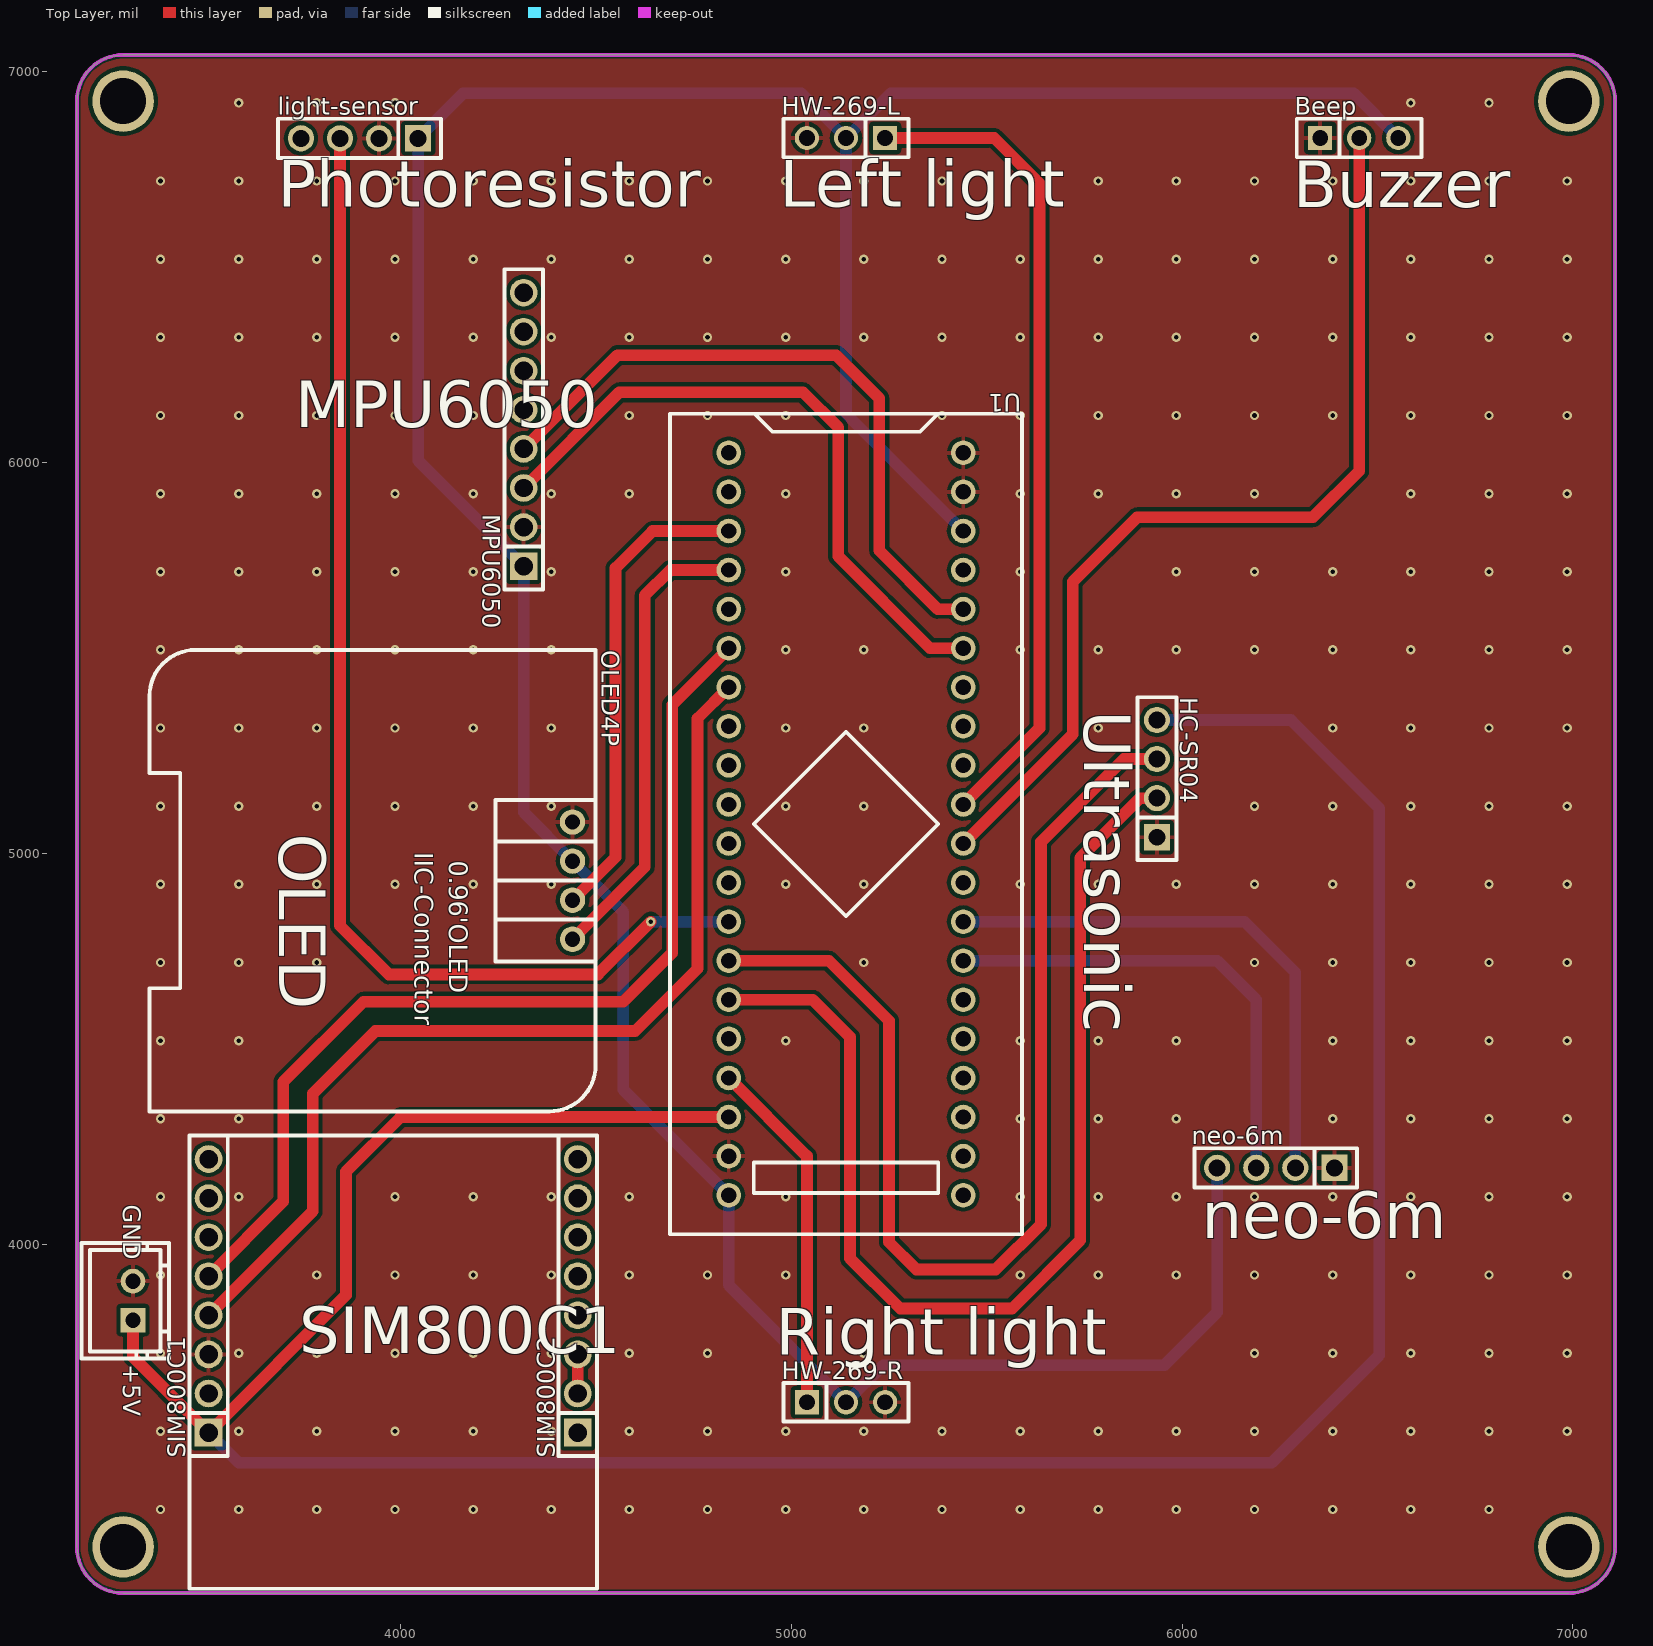
[diagram p0: Top Layer view]
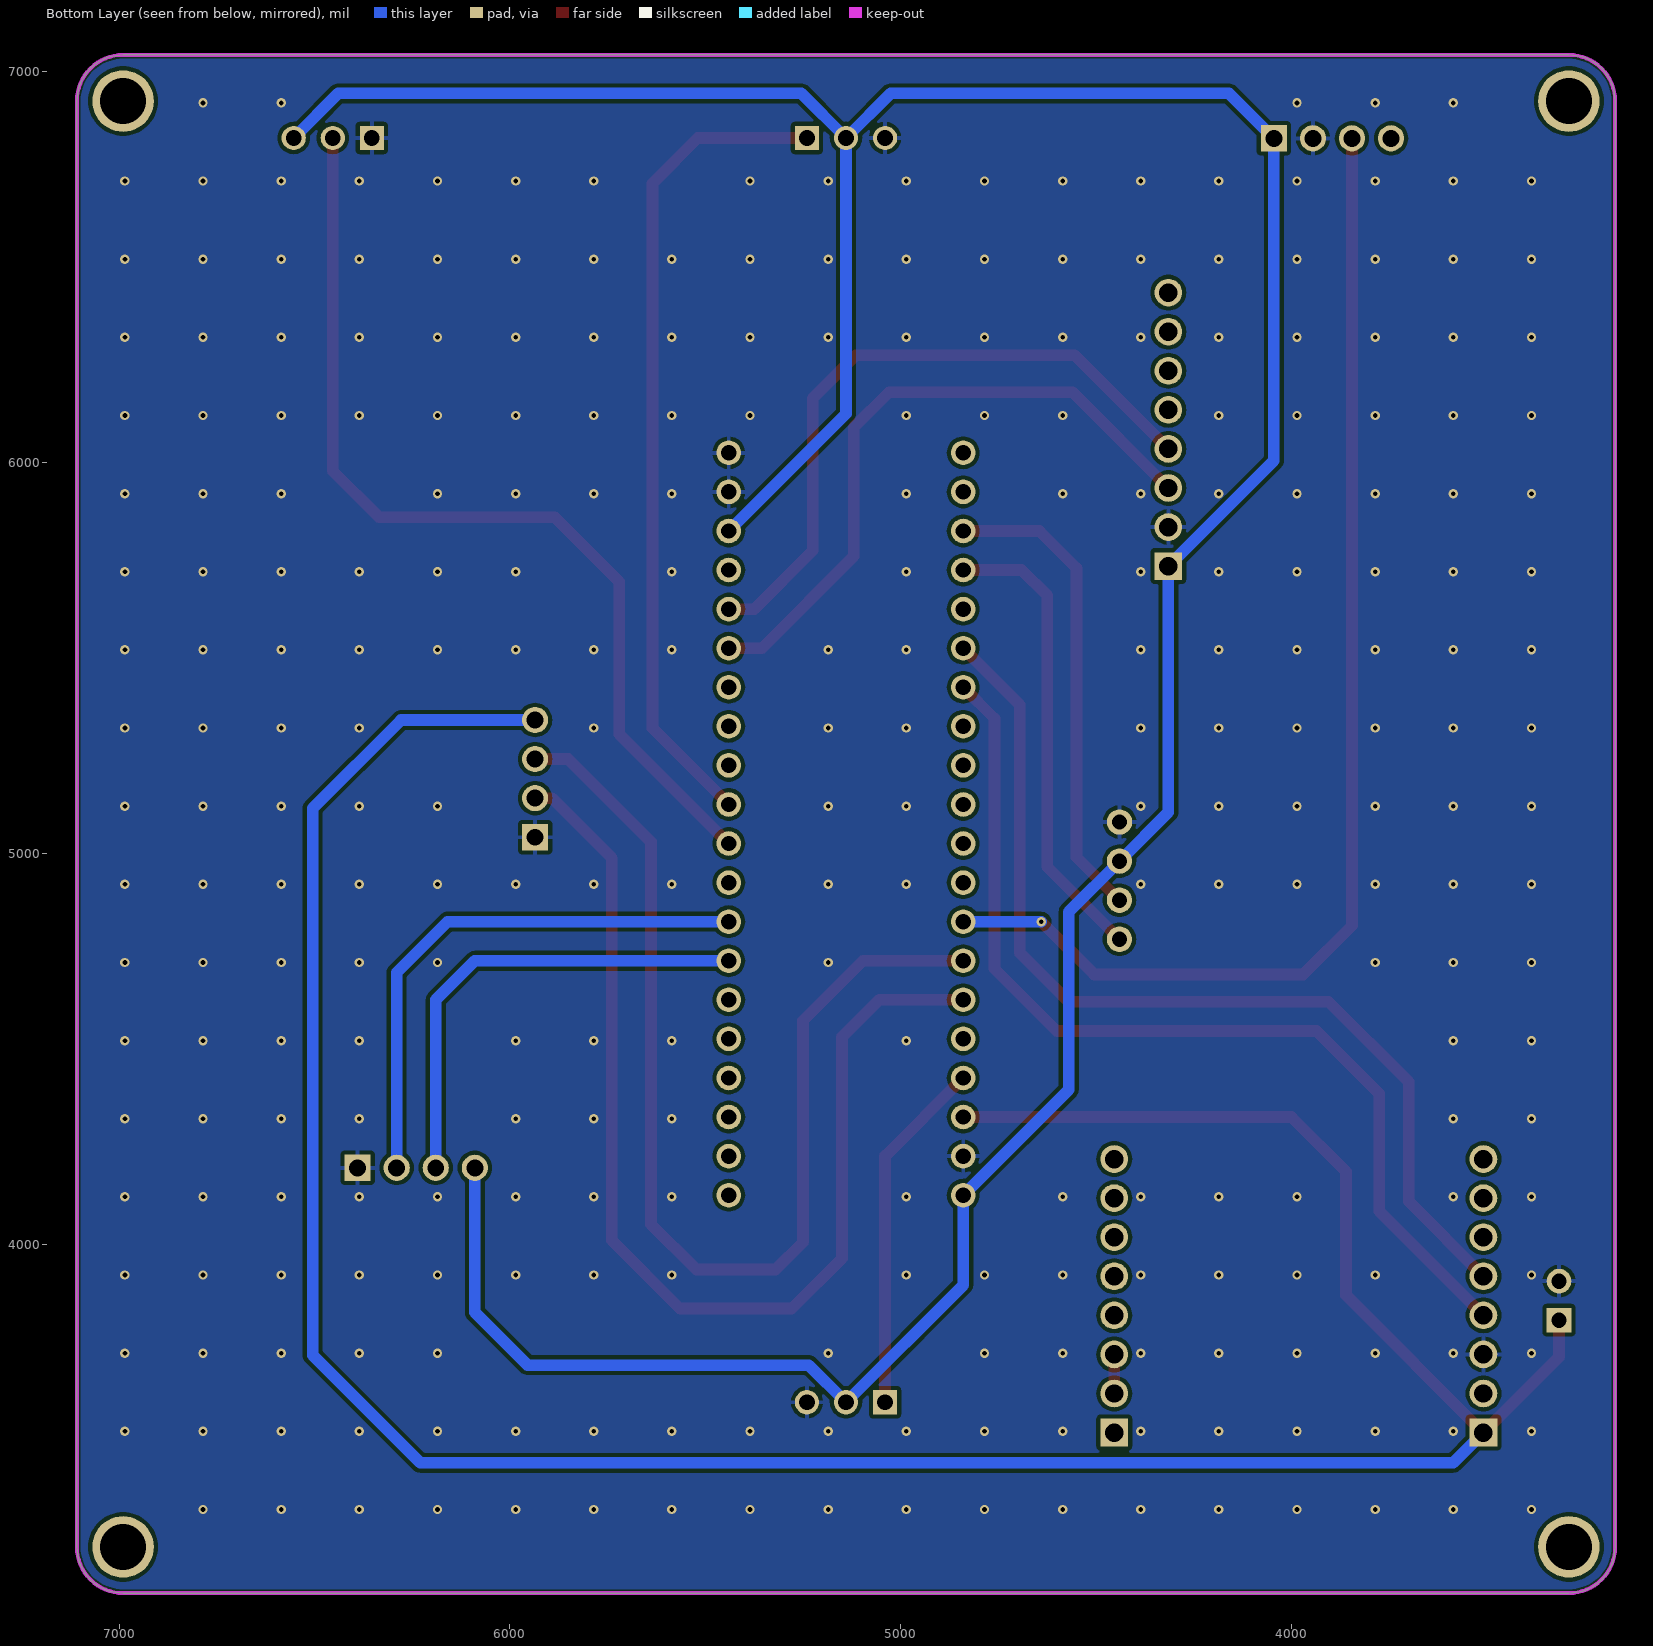
[diagram p1: Bottom Layer view, seen from below]
# Altium PCB MISC51587.pcbdoc
Units mil, origin at the board's own origin, x right, y up, seen from the top; angles counter-clockwise.
Board outline 3937.01 x 3937.01 mil, 2 copper layers (Top Layer, Bottom Layer), stack 62.206 mil thick; 12 components, 38 nets, 95 pads, 276 vias.

## Layer stack, top to bottom
Top Solder Mask Layer: solder mask 0.394, Dk 3.3
Top Layer: signal copper 1.379
Dielectric1: surface 59.449, FR4, Dk 4.5
Bottom Layer: signal copper 1.378
Bottom Solder Mask Layer: solder mask 0.394, Dk 3.3

## Board outline
6990.39,3106.5 ccw(c6990.39,3224.61) 7108.5,3224.61 7108.5,6925.39 ccw(c6990.39,6925.39) 6990.39,7043.5 3289.61,7043.5 ccw(c3289.61,6925.39) 3171.5,6925.39 3171.5,3224.61 ccw(c3289.61,3224.61) 3289.61,3106.5

## Design rules (kind name [scope] priority, off if disabled: settings)
BoardOutlineClearance copperThickness2oz_1 [All] p2 off: genericclearance=7.99 ignorepadtopadclearanceinfootprint=FALSE except(0: Arc-SplitContinuation Track-SplitContinuation SMDPad-SplitContinuation THPad-SplitContinuation Via-SplitContinuation Fill-SplitContinuation Region-SplitContinuation Poly-SplitContinuation Text-SplitContinuation Hole-SplitContinuation; 5.98: Arc-CutoutEdge Track-CutoutEdge SMDPad-CutoutEdge THPad-CutoutEdge Via-CutoutEdge Text-CutoutEdge; 6.89: Hole-OutlineEdge Hole-CutoutEdge; 10: Poly-OutlineEdge Poly-CutoutEdge; 11.81: Arc-OutlineEdge Track-OutlineEdge SMDPad-OutlineEdge THPad-OutlineEdge Via-OutlineEdge Fill-OutlineEdge Region-OutlineEdge Text-OutlineEdge Fill-CutoutEdge Region-CutoutEdge)
BoardOutlineClearance Plane_innerPlane_1 [All] p4 off: genericclearance=4.02 ignorepadtopadclearanceinfootprint=FALSE except(0: Arc-SplitContinuation Track-SplitContinuation SMDPad-SplitContinuation THPad-SplitContinuation Via-SplitContinuation Fill-SplitContinuation Region-SplitContinuation Poly-SplitContinuation Text-SplitContinuation Hole-SplitContinuation; 5.98: Arc-CutoutEdge Track-CutoutEdge SMDPad-CutoutEdge THPad-CutoutEdge Via-CutoutEdge Text-CutoutEdge; 6.89: Hole-OutlineEdge Hole-CutoutEdge; 10: Poly-OutlineEdge Poly-CutoutEdge; 11.81: Arc-OutlineEdge Track-OutlineEdge SMDPad-OutlineEdge THPad-OutlineEdge Via-OutlineEdge Fill-OutlineEdge Region-OutlineEdge Text-OutlineEdge Fill-CutoutEdge Region-CutoutEdge)
BoardOutlineClearance Copper_copperRegion_1 [All] p6 off: genericclearance=4.02 ignorepadtopadclearanceinfootprint=FALSE except(0: Arc-SplitContinuation Track-SplitContinuation SMDPad-SplitContinuation THPad-SplitContinuation Via-SplitContinuation Fill-SplitContinuation Region-SplitContinuation Poly-SplitContinuation Text-SplitContinuation Hole-SplitContinuation; 5.98: Arc-CutoutEdge Track-CutoutEdge SMDPad-CutoutEdge THPad-CutoutEdge Via-CutoutEdge Text-CutoutEdge; 6.89: Hole-OutlineEdge Hole-CutoutEdge; 10: Poly-OutlineEdge Poly-CutoutEdge; 11.81: Arc-OutlineEdge Track-OutlineEdge SMDPad-OutlineEdge THPad-OutlineEdge Via-OutlineEdge Fill-OutlineEdge Region-OutlineEdge Text-OutlineEdge Fill-CutoutEdge Region-CutoutEdge)
BoardOutlineClearance copperThickness1oz_1 [All] p8: genericclearance=4.02 ignorepadtopadclearanceinfootprint=FALSE except(0: Arc-SplitContinuation Track-SplitContinuation SMDPad-SplitContinuation THPad-SplitContinuation Via-SplitContinuation Fill-SplitContinuation Region-SplitContinuation Poly-SplitContinuation Text-SplitContinuation Hole-SplitContinuation; 5.98: Arc-CutoutEdge Track-CutoutEdge SMDPad-CutoutEdge THPad-CutoutEdge Via-CutoutEdge Text-CutoutEdge; 6.89: Hole-OutlineEdge Hole-CutoutEdge; 10: Poly-OutlineEdge Poly-CutoutEdge; 11.81: Arc-OutlineEdge Track-OutlineEdge SMDPad-OutlineEdge THPad-OutlineEdge Via-OutlineEdge Fill-OutlineEdge Region-OutlineEdge Text-OutlineEdge Fill-CutoutEdge Region-CutoutEdge)
Clearance copperThickness2oz [All] p1 off: gap=7.99 ignorepadtopadclearanceinfootprint=FALSE except(5.98: SMDPad-Track SMDPad-SMDPad THPad-Track SMDPad-THPad THPad-THPad Track-Via SMDPad-Via THPad-Via Via-Via Fill-SMDPad Region-SMDPad Fill-THPad Region-THPad Fill-Via Region-Via Fill-Fill Fill-Region Region-Region Arc-Track Arc-SMDPad Arc-THPad Arc-Via Fill-Arc Region-Arc Arc-Arc Text-Track SMDPad-Text Text-THPad Text-Via Fill-Text Region-Text Arc-Text Text-Text; 6.89: Hole-Track Hole-SMDPad Hole-THPad Hole-Via Fill-Hole Region-Hole Hole-Arc Hole-Text; 10: Poly-Track Poly-SMDPad Poly-THPad Poly-Via Poly-Fill Poly-Region Poly-Poly Poly-Arc Poly-Text Poly-Hole; 11.81: Fill-Track Region-Track)
Clearance Plane_innerPlane [All] p3 off: gap=4.02 ignorepadtopadclearanceinfootprint=FALSE except(5.98: SMDPad-Track SMDPad-SMDPad THPad-Track SMDPad-THPad THPad-THPad Track-Via SMDPad-Via THPad-Via Via-Via Fill-SMDPad Region-SMDPad Fill-THPad Region-THPad Fill-Via Region-Via Fill-Fill Fill-Region Region-Region Arc-Track Arc-SMDPad Arc-THPad Arc-Via Fill-Arc Region-Arc Arc-Arc Text-Track SMDPad-Text Text-THPad Text-Via Fill-Text Region-Text Arc-Text Text-Text; 6.89: Hole-Track Hole-SMDPad Hole-THPad Hole-Via Fill-Hole Region-Hole Hole-Arc Hole-Text; 10: Poly-Track Poly-SMDPad Poly-THPad Poly-Via Poly-Fill Poly-Region Poly-Poly Poly-Arc Poly-Text Poly-Hole; 11.81: Fill-Track Region-Track)
Clearance Copper_copperRegion [All] p5 off: gap=4.02 ignorepadtopadclearanceinfootprint=FALSE except(5.98: SMDPad-Track SMDPad-SMDPad THPad-Track SMDPad-THPad THPad-THPad Track-Via SMDPad-Via THPad-Via Via-Via Fill-SMDPad Region-SMDPad Fill-THPad Region-THPad Fill-Via Region-Via Fill-Fill Fill-Region Region-Region Arc-Track Arc-SMDPad Arc-THPad Arc-Via Fill-Arc Region-Arc Arc-Arc Text-Track SMDPad-Text Text-THPad Text-Via Fill-Text Region-Text Arc-Text Text-Text; 6.89: Hole-Track Hole-SMDPad Hole-THPad Hole-Via Fill-Hole Region-Hole Hole-Arc Hole-Text; 10: Poly-Track Poly-SMDPad Poly-THPad Poly-Via Poly-Fill Poly-Region Poly-Poly Poly-Arc Poly-Text Poly-Hole; 11.81: Fill-Track Region-Track)
Clearance copperThickness1oz [All] p7: gap=4.02 ignorepadtopadclearanceinfootprint=FALSE except(5.98: SMDPad-Track SMDPad-SMDPad THPad-Track SMDPad-THPad THPad-THPad Track-Via SMDPad-Via THPad-Via Via-Via Fill-SMDPad Region-SMDPad Fill-THPad Region-THPad Fill-Via Region-Via Fill-Fill Fill-Region Region-Region Arc-Track Arc-SMDPad Arc-THPad Arc-Via Fill-Arc Region-Arc Arc-Arc Text-Track SMDPad-Text Text-THPad Text-Via Fill-Text Region-Text Arc-Text Text-Text; 6.89: Hole-Track Hole-SMDPad Hole-THPad Hole-Via Fill-Hole Region-Hole Hole-Arc Hole-Text; 10: Poly-Track Poly-SMDPad Poly-THPad Poly-Via Poly-Fill Poly-Region Poly-Poly Poly-Arc Poly-Text Poly-Hole; 11.81: Fill-Track Region-Track)
DiffPairsRouting differentialPair [All] p1: maxlimit=6 minlimit=6 mostfreqgap=6 toplayer_minwidth=5 toplayer_prefwidth=10 toplayer_maxwidth=100 toplayer_mingap=6 toplayer_prefgap=6 toplayer_maxgap=6 bottomlayer_minwidth=5 bottomlayer_prefwidth=10 bottomlayer_maxwidth=100 bottomlayer_mingap=6 bottomlayer_prefgap=6 bottomlayer_maxgap=6 maxuncoupledlength=10
HoleToHoleClearance otherClearance [All] p1: gap=11.81 allowstackedmicrovias=TRUE
Length netLength [All] p1: minlimit=0 maxlimit=0
PasteMaskExpansion pasteMaskExpansion [All] p1: expansion=0
PlaneConnect innerPlane [All] p1: planeconnectstyle=Relief reliefexpansion=20 reliefentries=4 reliefconductorwidth=10 reliefairgap=10
PolygonConnect copperRegion [All] p1: connectstyle=Relief reliefconductorwidth=10 reliefentries=4 polygonreliefangle="90 Angle" airgapwidth=10 via.connectstyle=Relief via.reliefconductorwidth=10 via.reliefentries=4 via.polygonreliefangle="90 Angle" via.airgapwidth=10
RoutingVias viaSize [All] p1: holewidth=12.01 width=24.02 viastyle="Through Hole" minholewidth=11.81 minwidth=19.68 maxholewidth=248.03 maxwidth=393.7
SolderMaskExpansion solderMaskExpansion [IsVia] p1: expansion=-1000 istentingtop=TRUE
SolderMaskExpansion solderMaskExpansion [All] p2: expansion=2.01 istentingtop=FALSE
Width copperThickness2oz_2 [All] p1 off: maxlimit=100 minlimit=8 preferedwidth=10
Width copperThickness1oz_2 [All] p2: maxlimit=100 minlimit=5 preferedwidth=30

## Components (designator, comment, footprint, x,y, rotation, side; value= is the part's Value field where it differs from the comment)
+5V "_x001F_XH2.54-2P" CONN-TH_2P-P2.54-V 3315,3855 r90 top
Beep "" HDR-TH_3P-P2.54-V-F 6453.49,6830.79 r0 top
HC-SR04 "" HDR-TH_4P-P2.54-V-F 5935.69,5191.14 r90 top
HW-269-L "" HDR-TH_3P-P2.54-V-F 5140,6830.79 r180 top
HW-269-R "" HDR-TH_3P-P2.54-V-F 5140,3595 r0 top
light-sensor "" HDR-TH_4P-P2.54-V-F 3895,6830 r180 top
MPU6050 "" HDR-TH_8P-P2.54-V-F-1 4315,6085 r90 top
neo-6m "" HDR-TH_4P-P2.54-V-F 6240,4195 r180 top
OLED4P "" 0.96OLED_4P 4440,4930 r270 top
SIM800C1 "" HDR-TH_8P-P2.54-V-F-1 3508.5,3867.44 r90 top
SIM800C2 "" HDR-TH_8P-P2.54-V-F-1 4453.38,3867.44 r90 top
U1 "STM32F103C8T6-Card" CONN-TH_L53.3-W22.9_STM32F103C8T6-CARD 5140,5075 r270 top

## Footprints (in the part's own frame and the unit in brackets; to place one, negate y for a bottom-side part, rotate by r counter-clockwise, add the part's x,y. Pads: shape width x height; smd on the part's side, far side on the other; paste and mask are expansions set on the pad)
0.96OLED_4P [mm]
  round 1.65 hole 1 copper offset 0,0: 1(-3.81,-0.001) 2(-1.27,0.002) 3(1.27,0.002) 4(3.81,0.002)
  silkscreen extent -15,-27.5 15,1.5
CONN-TH_2P-P2.54-V [mm]
  rect 1.6x1.6 hole 1: 1(-1.27,0)
  round 1.6 hole 1: 2(1.27,0)
  silkscreen extent -3.75,-2.34 3.75,3.36
CONN-TH_L53.3-W22.9_STM32F103C8T6-CARD [mm]
  round 1.6 hole 1: 1(-24.13,-7.62) 2(-21.59,-7.62) 3(-19.05,-7.62) 4(-16.51,-7.62) 5(-13.97,-7.62) 6(-11.43,-7.62) 7(-8.89,-7.62) 8(-6.35,-7.62) 9(-3.81,-7.62) 10(-1.27,-7.62) 11(1.27,-7.62) 12(3.81,-7.62) 13(6.35,-7.62) 14(8.89,-7.62) 15(11.43,-7.62) 16(13.97,-7.62) 17(16.51,-7.62) 18(19.05,-7.62) 19(21.59,-7.62) 20(24.13,-7.62) 21(24.13,7.62) 22(21.59,7.62) 23(19.05,7.62) 24(16.51,7.62) 25(13.97,7.62) 26(11.43,7.62) 27(8.89,7.62) 28(6.35,7.62) 29(3.81,7.62) 30(1.27,7.62) 31(-1.27,7.62) 32(-3.81,7.62) 33(-6.35,7.62) 34(-8.89,7.62) 35(-11.43,7.62) 36(-13.97,7.62) 37(-16.51,7.62) 38(-19.05,7.62) 39(-21.59,7.62) 40(-24.13,7.62)
  silkscreen extent -26.67,-11.43 26.67,11.43
HDR-TH_3P-P2.54-V-F [mil]
  rect 62x62 hole 40.16: 1(-100,0)
  round 62 hole 40.16: 2(0,0) 3(100,0)
  silkscreen extent -160,-49 160,49
HDR-TH_4P-P2.54-V-F [mm]
  rect 1.7x1.7 hole 1.1: 1(-3.81,0)
  round 1.7 hole 1.1: 2(-1.27,0) 3(1.27,0) 4(3.81,0)
  silkscreen extent -5.29,-1.27 5.29,1.27
HDR-TH_8P-P2.54-V-F-1 [mm]
  rect 1.8x1.8 hole 1.2: 1(-8.89,0)
  round 1.8 hole 1.2: 2(-6.35,0) 3(-3.81,0) 4(-1.27,0) 5(1.27,0) 6(3.81,0) 7(6.35,0) 8(8.89,0)
  silkscreen extent -10.41,-1.25 10.41,1.25

## Free pads (board coordinates)
  round 157.48 hole 118.11: 1(3289.61,6925.39) 1(3289.61,3224.61) 1(6990.39,6925.39) 1(6990.39,3224.61)

## Via types
v1: diameter 24.02, hole 12, Top Layer to Bottom Layer, 276 vias

## Nets (pads, with @x,y where several pads share a name; then routed paths per layer and width w, separated by ;. In a path a pad name is that pad's centre, name@x,y a point inside that pad or via, vN(x,y) a via of type N, cw(c..) or ccw(c..) an arc to the next point about the centre after c; other vN are vias at no path point)
$1N18029: SIM800C2.2 SIM800C2.3 | length 100
  Top Layer w30: SIM800C2.2 SIM800C2.3
+5V: +5V.1 HC-SR04.4 SIM800C1.1 U1.18 | length 7424.3
  Top Layer w30: +5V.1 3315,3710.94 SIM800C1.1 3860,3868.94 3860,4185 4000,4325 U1.18
  Bottom Layer w30: SIM800C1.1 3585.94,3440 6230,3440 6505,3715 6505,5115 6278.86,5341.14 HC-SR04.4
GND: +5V.2 Beep.1 HC-SR04.1 HW-269-L.3 HW-269-R.3 light-sensor.2 MPU6050.2 neo-6m.1 OLED4P.1 SIM800C1.3 U1.19 U1.39 U1.40
  other v1: 3385.6,3320.6 3585.6,3320.6 3785.6,3320.6 3985.6,3320.6 4185.6,3320.6 4385.6,3320.6 4585.6,3320.6 4785.6,3320.6 4985.6,3320.6 5185.6,3320.6 5385.6,3320.6 5585.6,3320.6 5785.6,3320.6 5985.6,3320.6 6185.6,3320.6 6385.6,3320.6 6585.6,3320.6 6785.6,3320.6 3385.6,3520.6 3585.6,3520.6 3785.6,3520.6 3985.6,3520.6 4185.6,3520.6 4385.6,3520.6 4585.6,3520.6 4785.6,3520.6 4985.6,3520.6 5185.6,3520.6 5385.6,3520.6 5585.6,3520.6 5785.6,3520.6 5985.6,3520.6 6185.6,3520.6 6385.6,3520.6 6585.6,3520.6 6785.6,3520.6 6985.6,3520.6 3385.6,3720.6 3585.6,3720.6 3785.6,3720.6 3985.6,3720.6 4185.6,3720.6 4385.6,3720.6 4585.6,3720.6 4785.6,3720.6 5185.6,3720.6 6185.6,3720.6 6385.6,3720.6 6585.6,3720.6 6785.6,3720.6 6985.6,3720.6 3385.6,3920.6 3785.6,3920.6 3985.6,3920.6 4185.6,3920.6 4385.6,3920.6 4585.6,3920.6 4785.6,3920.6 4985.6,3920.6 5585.6,3920.6 5785.6,3920.6 5985.6,3920.6 6185.6,3920.6 6385.6,3920.6 6585.6,3920.6 6785.6,3920.6 6985.6,3920.6 3385.6,4120.6 3585.6,4120.6 3985.6,4120.6 4185.6,4120.6 4385.6,4120.6 4585.6,4120.6 4985.6,4120.6 5585.6,4120.6 5785.6,4120.6 5985.6,4120.6 6185.6,4120.6 6385.6,4120.6 6585.6,4120.6 6785.6,4120.6 6985.6,4120.6 3385.6,4320.6 3585.6,4320.6 5585.6,4320.6 5785.6,4320.6 5985.6,4320.6 6385.6,4320.6 6585.6,4320.6 6785.6,4320.6 6985.6,4320.6 3385.6,4520.6 3585.6,4520.6 4985.6,4520.6 5585.6,4520.6 5785.6,4520.6 5985.6,4520.6 6385.6,4520.6 6585.6,4520.6 6785.6,4520.6 6985.6,4520.6 3385.6,4720.6 3585.6,4720.6 3785.6,4720.6 5185.6,4720.6 6185.6,4720.6 6385.6,4720.6 6585.6,4720.6 6785.6,4720.6 6985.6,4720.6 3385.6,4920.6 3585.6,4920.6 3785.6,4920.6 3985.6,4920.6 4185.6,4920.6 4385.6,4920.6 4985.6,4920.6 5185.6,4920.6 5585.6,4920.6 5785.6,4920.6 5985.6,4920.6 6185.6,4920.6 6385.6,4920.6 6585.6,4920.6 6785.6,4920.6 6985.6,4920.6 3385.6,5120.6 3585.6,5120.6 3785.6,5120.6 3985.6,5120.6 4185.6,5120.6 4385.6,5120.6 4985.6,5120.6 5185.6,5120.6 6185.6,5120.6 6385.6,5120.6 6585.6,5120.6 6785.6,5120.6 6985.6,5120.6 3385.6,5320.6 3585.6,5320.6 3785.6,5320.6 3985.6,5320.6 4185.6,5320.6 4385.6,5320.6 4985.6,5320.6 5185.6,5320.6 5785.6,5320.6 6385.6,5320.6 6585.6,5320.6 6785.6,5320.6 6985.6,5320.6 3385.6,5520.6 3585.6,5520.6 3785.6,5520.6 3985.6,5520.6 4185.6,5520.6 4385.6,5520.6 4985.6,5520.6 5185.6,5520.6 5585.6,5520.6 5785.6,5520.6 5985.6,5520.6 6185.6,5520.6 6385.6,5520.6 6585.6,5520.6 6785.6,5520.6 6985.6,5520.6 3385.6,5720.6 3585.6,5720.6 3785.6,5720.6 3985.6,5720.6 4185.6,5720.6 4385.6,5720.6 4985.6,5720.6 5585.6,5720.6 5985.6,5720.6 6185.6,5720.6 6385.6,5720.6 6585.6,5720.6 6785.6,5720.6 6985.6,5720.6 3385.6,5920.6 3585.6,5920.6 3785.6,5920.6 3985.6,5920.6 4185.6,5920.6 4385.6,5920.6 4585.6,5920.6 4985.6,5920.6 5585.6,5920.6 5785.6,5920.6 5985.6,5920.6 6185.6,5920.6 6585.6,5920.6 6785.6,5920.6 6985.6,5920.6 3385.6,6120.6 3585.6,6120.6 3785.6,6120.6 3985.6,6120.6 4185.6,6120.6 4585.6,6120.6 4785.6,6120.6 4985.6,6120.6 5385.6,6120.6 5585.6,6120.6 5785.6,6120.6 5985.6,6120.6 6185.6,6120.6 6385.6,6120.6 6585.6,6120.6 6785.6,6120.6 6985.6,6120.6 3385.6,6320.6 3585.6,6320.6 3785.6,6320.6 3985.6,6320.6 4185.6,6320.6 4385.6,6320.6 4585.6,6320.6 4785.6,6320.6 4985.6,6320.6 5185.6,6320.6 5385.6,6320.6 5585.6,6320.6 5785.6,6320.6 5985.6,6320.6 6185.6,6320.6 6385.6,6320.6 6585.6,6320.6 6785.6,6320.6 6985.6,6320.6 3385.6,6520.6 3585.6,6520.6 3785.6,6520.6 3985.6,6520.6 4185.6,6520.6 4385.6,6520.6 4585.6,6520.6 4785.6,6520.6 4985.6,6520.6 5185.6,6520.6 5385.6,6520.6 5585.6,6520.6 5785.6,6520.6 5985.6,6520.6 6185.6,6520.6 6385.6,6520.6 6585.6,6520.6 6785.6,6520.6 6985.6,6520.6 3385.6,6720.6 3585.6,6720.6 3785.6,6720.6 3985.6,6720.6 4185.6,6720.6 4385.6,6720.6 4585.6,6720.6 4785.6,6720.6 4985.6,6720.6 5185.6,6720.6 5385.6,6720.6 5785.6,6720.6 5985.6,6720.6 6185.6,6720.6 6385.6,6720.6 6585.6,6720.6 6785.6,6720.6 6985.6,6720.6 3585.6,6920.6 3785.6,6920.6 3985.6,6920.6 6585.6,6920.6 6785.6,6920.6
NRST: U1.37
PA0: U1.25
PA1: U1.26
PA2: neo-6m.3 U1.27 | length 1221.4
  Bottom Layer w30: U1.27 6090,4725 6190,4625 neo-6m.3
PA3: neo-6m.2 U1.28 | length 1403.8
  Bottom Layer w30: U1.28 6160,4825 6290,4695 neo-6m.2
PA4: U1.29
PA5: Beep.2 U1.30 | length 2489.2
  Top Layer w30: U1.30 5720,5305 5720,5695 5885,5860 6335,5860 6453.49,5978.49 Beep.2
PA6: HW-269-L.1 U1.31 | length 2113.7
  Top Layer w30: HW-269-L.1 5519.21,6830.79 5635,6715 5635,5320 U1.31
PA7: U1.32
PA8: U1.5
PA9: SIM800C1.5 U1.6 | length 2548.6
  Top Layer w30: SIM800C1.5 3700,4108.94 3700,4415 3905,4620 4570,4620 4695,4745 4695,5380 U1.6
PA10: SIM800C1.4 U1.7 | length 2548.6
  Top Layer w30: SIM800C1.4 3775,4083.94 3775,4385 3935,4545 4600,4545 4760,4705 4760,5345 U1.7
PA11: U1.8
PA12: U1.9
PA15: U1.10
PB0: U1.33
PB1: U1.34
PB3: U1.11
PB4: U1.12
PB5: light-sensor.3 U1.13 | length 3117.7
  Top Layer w30: light-sensor.3 3845,4815 3970,4690 4505,4690 v1(4640,4825)
  Bottom Layer w30: v1(4640,4825) U1.13
PB6: HC-SR04.3 U1.14 | length 2869.2
  Top Layer w30: U1.14 5096.42,4725 5250,4571.42 5250,4005 5320,3935 5523.58,3935 5639.29,4050.71 5639.29,5029.62 5850.81,5241.14 HC-SR04.3
PB7: HC-SR04.2 U1.15 | length 2869.2
  Top Layer w30: U1.15 5055,4625 5150,4530 5150,3963.58 5278.58,3835 5565,3835 5739.29,4009.29 5739.29,4988.2 5892.23,5141.14 HC-SR04.2
PB8: U1.16
PB9: HW-269-R.1 U1.17 | length 912.8
  Top Layer w30: U1.17 5040,4225 HW-269-R.1
PB10: MPU6050.3 U1.35 | length 1691.1
  Top Layer w30: MPU6050.3 4560,6180 5030,6180 5120,6090 5120,5760 5355,5525 U1.35
PB11: MPU6050.4 U1.36 | length 1722.1
  Top Layer w30: MPU6050.4 4555,6275 5115,6275 5225,6165 5225,5775 5375,5625 U1.36
PB12: U1.1
PB13: U1.2
PB14: OLED4P.3 U1.3 | length 1224.9
  Top Layer w30: OLED4P.3@4440.05,4880 4550,4989.95 4550,5730 4645,5825 U1.3
PB15: OLED4P.4 U1.4 | length 1198.5
  Top Layer w30: OLED4P.4@4440.05,4780 4625,4964.95 4625,5660 4690,5725 U1.4
PC13: U1.22
PC14: U1.23
PC15: U1.24
VBAT: U1.21
VCC: Beep.3 HW-269-L.2 HW-269-R.2 light-sensor.1 MPU6050.1 neo-6m.4 OLED4P.2 U1.20 U1.38 | length 8931.9
  Bottom Layer w30: U1.38 5140,6125 HW-269-L.2 ; neo-6m.4 6090,3825 5955,3690 5235,3690 HW-269-R.2 4840,3895 U1.20 4570,4395 4570,4850.05 4440.05,4980 4315,5105.05 MPU6050.1 4045,6005 light-sensor.1 4160,6945 5025.79,6945 HW-269-L.2 ; Beep.3 6439.28,6945 5254.21,6945 HW-269-L.2
pads on no net: light-sensor.4 MPU6050.5 MPU6050.6 MPU6050.7 MPU6050.8 SIM800C1.2 SIM800C1.6 SIM800C1.7 SIM800C1.8 SIM800C2.1 SIM800C2.4 SIM800C2.5 SIM800C2.6 SIM800C2.7 SIM800C2.8

## Polygon pours and split planes (outlines as drawn)
GND on Bottom Layer (solid, remove dead copper, pour order 2): 3100,7165 3100,3000 7275,3000 7275,7165
GND on Top Layer (solid, remove dead copper, pour order 0): 3000,7145 3000,3075 7385,3075 7385,7145

## Keep-outs
Board Outline Layer:
  the board outline again, w10

## Silkscreen, mask and mechanical layers (free items; w line width, h text height)
Top Silkscreen Layer:
  lines w10: 3459.29,3117.6 3459.29,4277.28 4502.6,4277.28 4502.6,3117.6 3459.29,3117.6
  text "Photoresistor" at 3685,6655 h120
  text "Left light" at 4970,6655.18 h120
  text "Buzzer" at 6285,6654.09 h120
  text "MPU6050" at 3730,6090 h120
  text "Ultrasonic" at 5750,5365 h120 r270
  text "OLED" at 3689.69,5050 h120 r270
  text "GND" at 3290,4100 h45 r270
  text "neo-6m" at 6050,4015 h120
  text "SIM800C1" at 3740,3720 h120
  text "Right light" at 4960,3716.14 h120